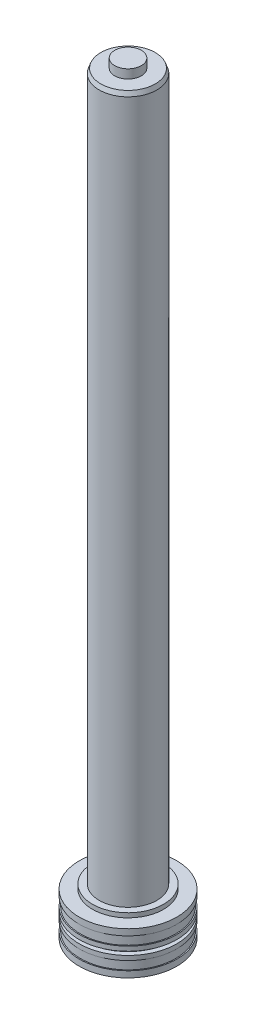
SolidWorks part; units mm, degrees
material "AISI 1045 钢，冷拔"
ref_plane "Front Plane" through (0, 0, 0) normal (0, 0, 1) x (1, 0, 0)
ref_plane "Top Plane" through (0, 0, 0) normal (0, 1, 0) x (1, 0, 0)
ref_plane "Right Plane" through (0, 0, 0) normal (1, 0, 0) x (0, 0, -1)
sketch "Sketch1" plane through (0, 0, 0) normal (0, 0, 1) x (1, 0, 0)
  line L0 (0, 0) -> (0, 487.9716) construction
  line L1 (0, 0) -> (80, 0)
  line L2 (80, 0) -> (80, 9.9)
  line L3 (80, 9.9) -> (110, 9.9)
  line L4 (110, 9.9) -> (110, 23.9)
  line L5 (110, 23.9) -> (107.5, 23.9)
  line L6 (107.5, 23.9) -> (107.5, 43.9)
  line L7 (107.5, 43.9) -> (110, 43.9)
  line L8 (110, 43.9) -> (110, 53.9)
  line L9 (110, 53.9) -> (99.5, 53.9)
  line L10 (99.5, 53.9) -> (99.5, 62)
  line L11 (99.5, 62) -> (110, 62)
  line L12 (110, 62) -> (110, 72)
  line L13 (110, 72) -> (107.5, 72)
  line L14 (107.5, 72) -> (107.5, 92)
  line L15 (107.5, 92) -> (110, 92)
  line L16 (110, 92) -> (110, 106)
  line L17 (110, 106) -> (80, 106)
  line L18 (65, 116) -> (65, 1698)
  line L19 (61.3603, 1708) -> (30, 1708)
  line L20 (30, 1708) -> (30, 1728)
  line L21 (30, 1728) -> (0, 1728)
  line L22 (0, 1728) -> (0, 0)
  line L23 (151.7911, 0) -> (0, 0) construction
  line L24 (0, 0) -> (0, -20.8959) construction
  line L25 (65, 116) -> (80, 116)
  line L26 (80, 116) -> (80, 106)
  line L27 (61.3603, 1708) -> (65, 1698)
  dimension "D2" = 1728
  dimension "D3" = 20
  dimension "D4" = 14
  dimension "D5" = 20
  dimension "D6" = 10
  dimension "D7" = 8.1
  dimension "D8" = 10
  dimension "D9" = 20
  dimension "D10" = 116
  dimension "D11" = 60
  dimension "D12" = 130
  dimension "D13" = 220
  dimension "D14" = 199
  dimension "D15" = 2.5
  dimension "D16" = 30
  dimension "D17" = 160
  dimension "D18" = 1592
  dimension "D19" = 160
  dimension "D20" = 10
  dimension "D21" = 14
  dimension "D22" = 215
  dimension "D23" = 9.9
  dimension "D24" = 10
  dimension "D25" = 20
revolve "Revolve1" add sketch "Sketch1" angle 360 about L0
